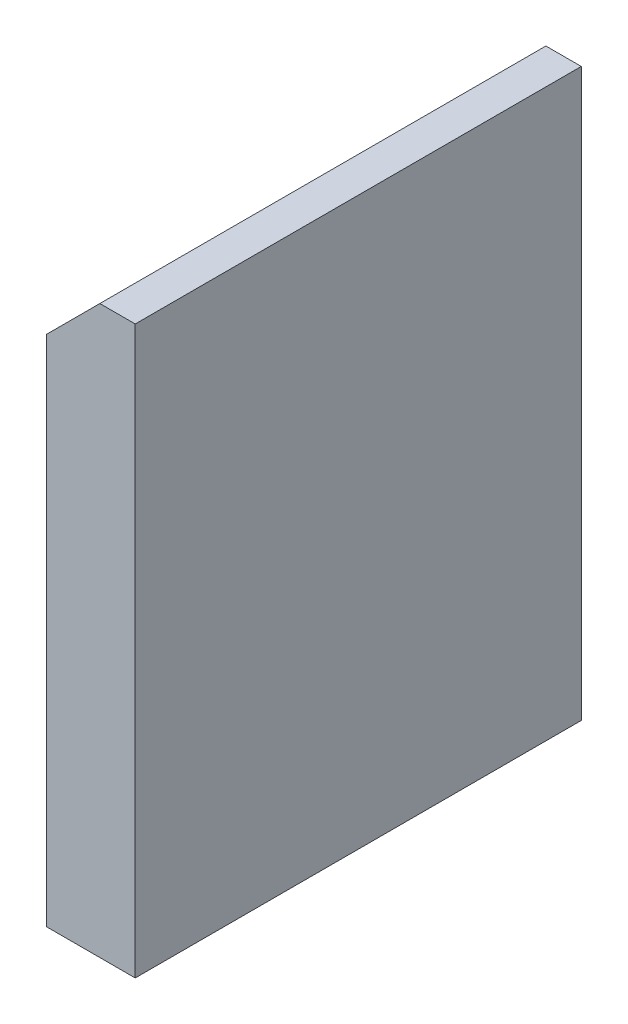
from build123d import *

# Parameters (mm, degrees)
SKETCH2_W           = 25
SKETCH2_H           = 126
BOSS_EXTRUDE1_DEPTH = 80
CHAMFER1_SIZE       = 15


with BuildPart() as part:
    # Sketch2 → Boss-Extrude1 (new, symmetric)
    with BuildSketch(Plane(origin=(0, 0, 0), x_dir=(1, 0, 0), z_dir=(0, 1, 0))):
        Rectangle(SKETCH2_W, SKETCH2_H)
    extrude(amount=BOSS_EXTRUDE1_DEPTH, both=True)

    # Chamfer1
    chamfer1_edges = [part.edges().sort_by_distance(p)[0] for p in [
        (-12.5, 80, 0),
    ]]
    chamfer(chamfer1_edges, length=CHAMFER1_SIZE)


solid = part.part
